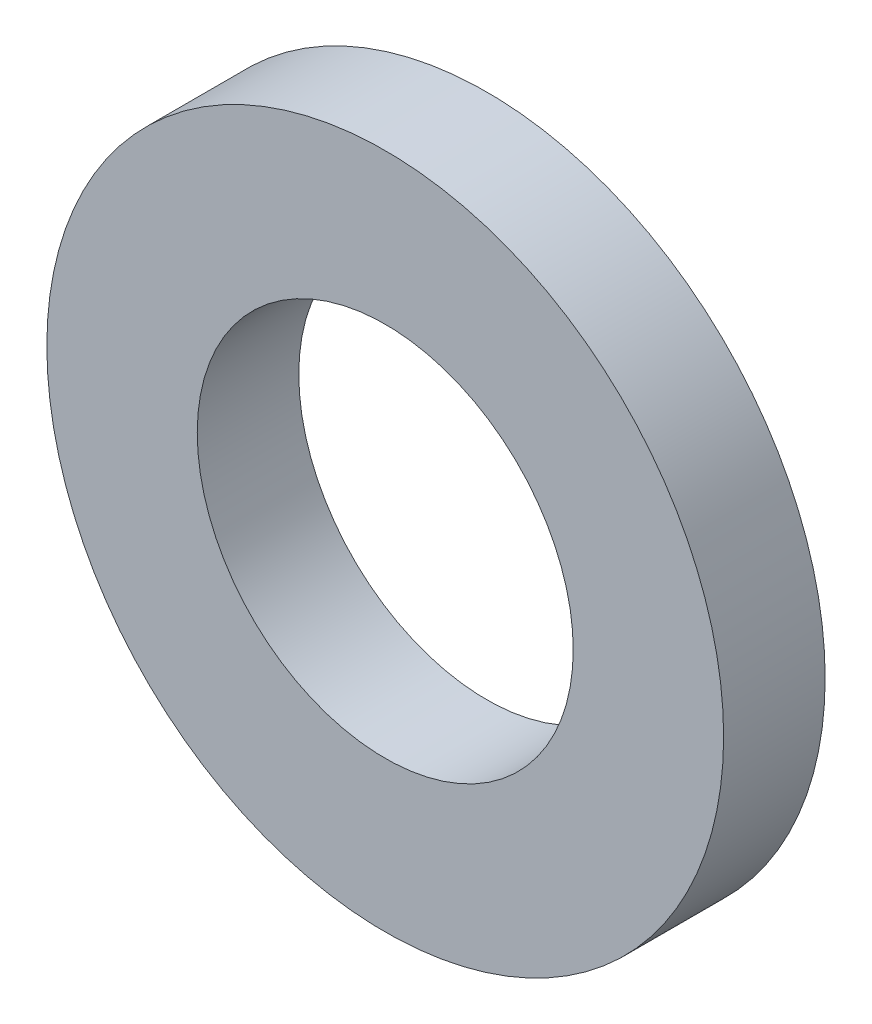
from build123d import *

# Parameters (mm, degrees)
SKETCH1_R           = 9
SKETCH1_R_2         = 5
BOSS_EXTRUDE1_DEPTH = 2.7


with BuildPart() as part:
    # Sketch1 → Boss-Extrude1 (new body)
    with BuildSketch(Plane.XY):
        with Locations(Location((0, 0, 0), (0, 0, 180))):
            Circle(SKETCH1_R)
        with Locations(Location((0, 0, 0), (0, 0, 180))):
            Circle(SKETCH1_R_2, mode=Mode.SUBTRACT)
    extrude(amount=BOSS_EXTRUDE1_DEPTH)


solid = part.part
